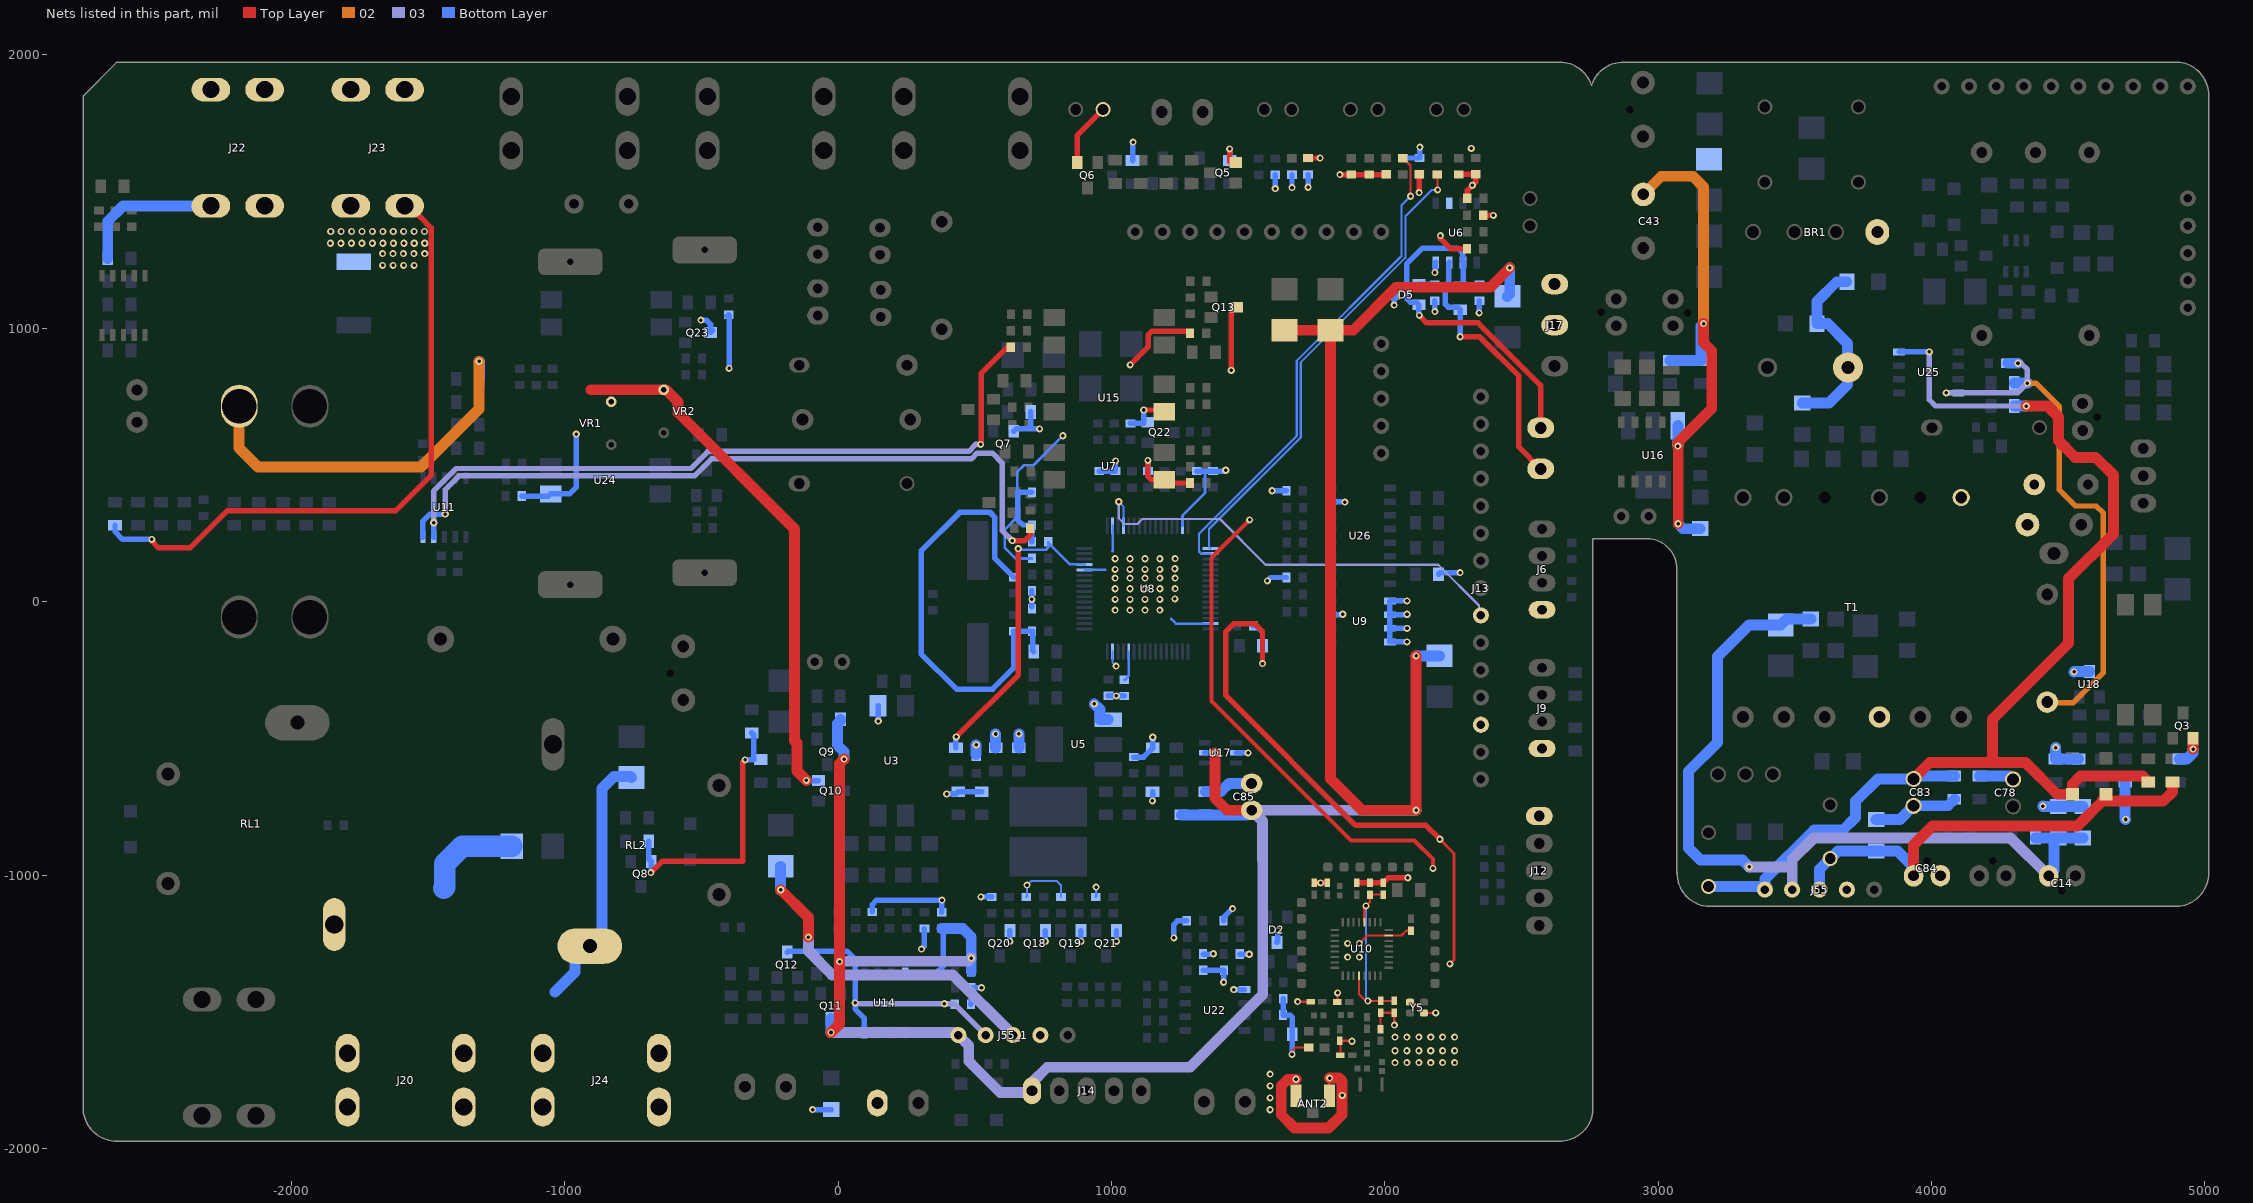
[diagram p0: the nets of this part, all layers, seen from the top]
# Altium PCB MISC105418.PcbDoc (part 3 of 7)
Units mil, origin at the board's own origin, x right, y up, seen from the top; angles counter-clockwise.
Board outline 7774.32 x 3947.04 mil, 4 copper layers (Top Layer, 02, 03, Bottom Layer), stack 30.635 mil thick; 459 components, 285 nets, 1258 pads, 468 vias.
Unrouted connection lines stored in the file: 23.

## Part data
ANT1: library part 天线
BR1: library part BRIDGE1, "Diode Bridge"
C1 C2 C3 C5 C7 C8 C9 C10 C11 C12 C25 C27 C28 C29 C30 C31 C33 C44 C49 C79 C80 C81 C82 C86 C87 C119 C120 CX2 CY1: library part CAP, "Capacitor"
C4 C37 C41 C50 C54 C55 C56 C57 C58 C59 C61 C63 C64 C65 C66 C67 C68 C69 C70 C71 C72 C73 C77 C90 C91 C92 C93 C95 C96 C97 C103 C104 C105 C106 C109 C115 C116 C117 C118: library part CAP/0805, "0.1uF, ,X7R, 10%,50V, SMD"
C6 C13 C14 C36 C43 C62 C78 C83 C84 C85: library part ELECTRO1, "Electrolytic Capacitor"
C15 C20 C22 C26 C32 C40 C45 C46 C48 C111 C125 C127: library part C0805, "0.1uF/50V, X7R,10%, SMD"
C17 C18 C19 C23: library part "Cap Semi", "1uF/50V, X7R,10%, SMD"
C21 C107 C108: library part CAP/0805, "10uF/10V, X7R, 10%,SMD"
C24 C88 C89: library part C0805, "15pF/50V, X7R,10%, SMD"
C38 C101 C112 C123 C124 C129: library part C0805, "1uF/50V, X7R,10%, SMD"
C39 C110: library part C0805, "20pF/50V, X7R,10%, SMD"
C42 C47: library part ELECTRO
C51: library part C0805
C60: library part CAP/0805, "18pF, ,X7R, 10%,50V, SMD"
C74 C76: library part CAP/0603, "0603 SMD ceramic capacitor/ generic footprint"
C98 C99 C100: library part CAP/0805, "33nF, X7R, 10%,SMD"
C102: library part C0805, "2.2uF/50V, X7R,10%, SMD"
C114: library part C0805, "1nF/50V, X7R,10%, SMD"
C121: library part CAP/EC10B, "Electrolytic capacitor 6.8uF/400V / 20% / DIP / horizontal"
CX1: library part CAP_X2, "X capacitor-275AC-224K"
CX3: library part CAP
D2 D5: library part NUP2105L, "NUP2105L,SMD"
D3 D4 D9 D11: library part DIODE
D6 D7 D8 D10 D14 D15 D16 D19 D20 D21 D22 D23 D25 D26 D555: library part DIODE1, "Diode"
D12 D13: library part Diode/SMD2, "SMD diode, 1N4148"
D17 D31: library part Diode/SMD3, "SMD diode: 1N4148"
D24: library part DIODE, "Diode"
D29 D30: library part Diode/SMD2, "SMD diode, US1M"
F1: library part FUSE2, "Fuse"
FB1: library part L3*3*1.5, "SMD ferrite bead"
FB2: library part Inductor
J1 J2 J3 J4 J25: "Connector/2.54mm pitch/1 X 2"
J6 J9: library part XHS-4, "Connector/2.54mm pitch/1 X 4"
J7 J8 J16 J26: library part XHS-2, "Connector/3.81mm pitch/1 X 2"
J11 J20 J21 J22 J23 J24 J28 J29: "Cord connector"
J12 J14: "2.54mm pin header"
J13: library part Header-15,2.54mm, "Header-15,2.54mm"
J15: "Connector/3.81mm pitch/1 X 2"
J55 J55_1 P51 P51_1: library part Header-5.2.54mm, "Header-5.2.54mm"
L1: library part "Ind DR 10x12"
L11 L21 L22 L31: library part L3*3*1.5
L24 L25 L29: library part "INDUCTOR IRON"
L26 L27 L28 L30: library part L3*3*1.5, "SMD inductor"
LF1: library part TRANS6
Q1 Q3: library part NPN1, "NPN Transistor"
Q2: library part "MOSFET N"
Q5 Q6 Q7 Q8 Q10: library part 2N7002, "N-Channel ,AP2306AGN"
Q9 Q14 Q16: library part MOS管P沟道SMD, "P-Channel ,AOSS21311C"
Q11: library part Q-NPN
Q12: library part Q-PNP
Q18 Q19 Q20 Q21 Q22: library part MOS管N沟道SMD, "N-Channel ,AP2306AGN"
R5 R8 R10 R12 R13 R14 R16 R17 R19 R20 R22 R23 R241: library part RES1
R6 R7 R9 R11 R15 R21 R24 R25 R26 R27 R28 R29 R32 R33 R35 R36 R37: library part RES2A, "Resistor"
R18 R141 R142 R156 R159: library part RES/0603
R30 R31 R34: library part RE2A
R38 R39 R45 R88 R92 R95: library part "R 1206_Dup1"
R40 R47 R48 R51 R60 R83 R87 R93 R105 R127 R134 R137 R170 R174 R175 R177 R234 R235 R236 R238: library part RES/0603, "100R,1%,1/10W,SMD"
R41 R125 R126 R213 R214: library part RES/0603, "5.1K,1%,1/10W,SMD"
R42 R43 R113 R114 R116 R117 R119 R120 R121 R122 R151 R153 R155 R157 R158: library part RES/0603, "1K,1%,1/10W,SMD"
R44: library part RES/0805, "1M,1%,1/10W,SMD"
R46 R49 R50 R52 R53 R54 R55 R77 R115 R118 R128 R147 R150 R152 R154 R162 R163 R171 R173 R178 R189 R190 R233 R239 R240 R264: library part RES/0603, "10K,1%,1/10W,SMD"
R56 R57: library part RES/0603, "1K,1%,1/8W,SMD"
R58 R59 R68 R69 R73 R74 R130 R136: library part RES/0603, "10K,1%,1/8W,SMD"
R61 R64 R80 R86 R90 R104 R108 R111 R133: library part RES/0603, "4.7K,1%,1/10W,SMD"
R63 R66 R89 R107 R110: library part RES/0805, "300R,1%,1/8W,SMD"
R65 R85 R91 R109 R112: library part RES/0603, "2K,1%,1/10W,SMD"
R67 R71 R72: library part RES/0603, "470R,1%,1/8W,SMD"
R70 R129 R135: library part RES/0603, "5.1K,1%,1/8W,SMD"
R75: library part RES/0805, "2K,1%,1/8W,SMD"
R78: library part RES/0603, "120K,1%,1/10W,SMD"
R79: library part RES/0603, "1.5K,1%,1/10W,SMD"
R81 R82: library part RES/0603, "20K,1%,1/10W,SMD"
R84: library part RES/0603, "100K,1%,1/10W,SMD"
R94 R102 R185 R186 R187 R231: library part RES/0805, "1.5M,5%,1/8W,SMD"
R96: library part RES/0805, "0R,1%,1/8W,SMD"
R97 R99 R182 R183 R184 R188: library part RES/0805, "1K,1%,1/8W,SMD"
R100: library part RES/0805, "510K,1%,1/8W,SMD"
R103: library part RES/0805, "NC"
R123 R124 R145: library part RES/0805, "3K,5%,1/8W,SMD"
R139 R140 R260 R261: library part RES/0603, "0R,1%,1/10W,SMD"
R148 R149 R191 R192 R193 R194 R197 R199 R201: library part "Res Semi", "Semiconductor Resistor"
R176 R179: library part RES/0603, "100R,1%,1/8W,SMD"
R180 R181: library part RES/0603, "100R,5%,1/8W,SMD"
R195 R198 R200 R263: library part RES/0603, "30K,1%,1W,SMD"
R196: library part RES/0805, "10K, 5%,1/8W, SMD"
R232: library part RES/0805, "1K,5%,1/8W,SMD"
R237: library part RES/0603, "3K,1%,1/10W,SMD"
RL1 RL2: library part HF33F05HSL
RNTC1 RNTC2: library part RES/VARISTOR
T1: library part PQ2020
T2: library part "IND CM T6x3x2"
U1: library part OB2365
U2 U3 U7 U15 U23 U24: library part TLP521-1
U5 U16: library part CM1117, "CM1117"
U9: library part 24LC128
U12: library part DHC05CD4
U14: library part SGM8272, "LM358"
U17: "SM8102H, Pin to Pin"
U18: "Zener Diode"
U20: library part OPTO2A, "Optoisolator"
U22: library part ADM483E
U25: library part LM393D, "Dual Comparator"
U26: library part MAX232ACSE, "+5V Powered, Multi-Channel RS-232 Driver/Receiver"
VR1 VR2: library part RES/VARISTOR, "Varistor, TFMOV10M250"
Y1 Y5: library part CS325
Y2 Y3: library part CAP_X2, "10nF/2KV, X7R, 10%,SMD"
ZC1: library part 放电管
ZD1: library part ZENER1, "Zener Diode"
ZD2 ZD3: library part ZENER2, "Zener Diode"

## Free pads (board coordinates)
  oval 133.86x157.48 hole 125.98: 1(-2191,-56.5) 1(-2191,715) 1(-1932,-56.5) 1(-1932,715)

## Via types
v1: diameter 26, hole 13, Top Layer to Bottom Layer, tented both sides, 468 vias

## Nets (pads, with @x,y where several pads share a name; then routed paths per layer and width w, separated by ;. In a path a pad name is that pad's centre, name@x,y a point inside that pad or via, vN(x,y) a via of type N, cw(c..) or ccw(c..) an arc to the next point about the centre after c; other vN are vias at no path point)
1V2: C102.2 C111.1 C112.1 C127.2 U10.12 U10.28 | length 714.5
  Top Layer w8: U10.28@1905.25,-1368.92 1905.25,-1436.25 1929.79,-1460.79 v1(1938,-1460.79) C111.1@1984.76,-1460.79 C112.1@2034.17,-1460.79 ; U10.12@1924.94,-1172.07 1924.94,-1119.06 v1(1931,-1113) 1945.43,-1098.57 C127.2@1945.43,-1071.49 C102.2@1993.76,-1071.49
  Bottom Layer w8: v1(1931,-1113) 1931,-1453.79 v1(1938,-1460.79)
4GEN/SPI-CS-PA4: J13.9 U8.20 | length 1659.4
  03 w8: v1(1026.47,365.47) 1026.47,304.53 1047,284 1095,284 1113,302 1396.6,302 1563.6,135 2195.18,135 2344.42,-14.24 2344.42,-43.63 J13.9@2351.09,-50.3
  Bottom Layer w8: v1(1026.47,365.47) 1043.51,348.43 U8.20@1043.51,277.82
12VA: C43.1 C44.2 D9.1 L1.2 R95.1 U16.3 | length 1975.7
  Top Layer w39.37: v1(3073,285) 3073,568 v1(3072,569) 3072,582.76 3196,706.76 3196,917.42 3166,947.42 v1(3166,1017)
  02 w39.37: C43.1@2945.36,1490.03 3011.33,1556 3127,1556 3166,1517 v1(3166,1017)
  Bottom Layer w19.68: v1@3071.95,569.05 v1(3072,569)
  Bottom Layer w39.37: L1.2@3042.88,882.44 C44.2@3156,882.44 3156,1007 v1(3166,1017) ; v1@3071.95,569.05 U16.3@3071.95,644.04 ; v1(3073,285) 3091.04,266.96 R95.1@3154,266.96
+6V: C84.1 D15.1 J55.3 J55_1.3 L25.2 R26.1 R34.2 ZD2.2 | length 2907.9
  Top Layer w40: v1(-210,-1054) -109,-1155 v1(-109,-1227) ; C84.1@3934.06,-1002.89 3934.06,-889.94 4003,-821 4533,-821 4624,-730 4847,-730 4881,-696 R26.1@4881,-659.32
  03 w40: v1(-109,-1227) -109,-1278 -22,-1365 419.07,-1365 J55_1.3@639.81,-1585.74
  Bottom Layer w40: v1(-210,-1054) D15.1@-210,-967.8 ; J55.3@3590.09,-1053.5 3590.09,-978.92 L25.2@3629.09,-939.92 3656.96,-912.06 R34.2@3797.09,-912.06 3875.35,-912.06 3934.06,-970.76 C84.1@3934.06,-1002.89
+12.7V: C46.2 C83.1 C85.1 C86.2 C87.2 D7.1 D8.1 D16.1 D555.1 J14.1 J55.1 J55_1.1 L24.2 Q9.2 Q11.3 R28.1 R35.1 R70.1 R75.1 R77.2 R194.1 U14.8 U17.5 U25.8 ZD3.2 | length 14291.5
  Top Layer w39.37: v1(-26,-1576) 5.32,-1544.68 v1(5.32,-1316.88) 5.32,-592.68 v1(22,-576) ; D8.1@1633,993.2 D16.1@1801,993.2 1884.2,993.2 2041,1150 2386,1150 v1(2457,1221)
  Top Layer w40: v1(1379,-553) 1379,-719 1423,-763 C85.1@1513,-763 ; D16.1@1801,993.2 1801,-648 1916,-763 v1(2114,-763) 2114.5,-762.5 v1(2114.5,-198.5) ; C83.1@3933.98,-648.28 3993.26,-589 4206,-589 ; v1(4346,715.53) 4423.47,715.53 4464,675 4464,589 4525,528 4600,528 4665,463 4665,248 4501,84 4501,-152 4223.49,-429.51 4223.49,-571.51 4206,-589 ; R28.1@4793,-659.32 4771.68,-638 4545,-638 4515.09,-667.91 ZD3.2@4515.09,-704.5 4459.39,-704.5 4343.89,-589 4206,-589
  03 w19.68: v1(3991.5,913.5) 3991.5,738.5 4014.47,715.53 v1(4346,715.53)
  03 w39.37: v1(-26,-1576) 430.07,-1576 J55_1.1@439.81,-1585.74 478,-1623.93 478,-1681.33 592.67,-1796 702.47,-1796 J14.1@708.98,-1789.5 708.98,-1759.02 765,-1703 1287,-1703 1553,-1437 1553,-947 ; v1@7.2,-1315 475.94,-1315 v1(486.94,-1304)
  03 w40: 1553,-947 1553,-803 C85.1@1513,-763 v1(2114,-763)
  Bottom Layer w19.68: U25.8@3880.83,913.5 v1(3991.5,913.5)
  Bottom Layer w20: U14.8@245.09,-1359.23 358.77,-1359.23 385,-1333 385,-1201.72 C46.2@378.89,-1195.61 ; U17.5@1340.91,-553 v1(1379,-553)
  Bottom Layer w39.37: v1(-26,-1576) -25.91,-1575.91 Q11.3@-25.91,-1525.22 ; R75.1@5.32,-1360.82 v1(5.32,-1316.88) ; R70.1@8.32,-430 8.32,-435.31 -2.6,-446.24 Q9.2@-2.6,-502.74 -2.6,-524.91 22,-549.5 v1(22,-576) ; C46.2@378.89,-1195.61 455.61,-1195.61 486.94,-1226.94 v1(486.94,-1304) R77.2@486.94,-1353.53 ; D7.1@2448.09,1116.5 2457,1125.41 v1(2457,1221)
  Bottom Layer w40: R35.1@1255.09,-779.82 C86.2@1343.09,-779.82 1496.18,-779.82 C85.1@1513,-763 ; v1(2114.5,-198.5) D555.1@2200.09,-198.5 ; L24.2@3184.09,-1041.92 3378.52,-1041.92 J55.1@3390.09,-1053.5 3390.09,-1014.91 3569,-836 3675,-836 3722,-789 3722,-730 3803.72,-648.28 C83.1@3933.98,-648.28 3944.09,-638.17 C87.2@4083.09,-638.17 ; R194.1@4302.22,715.53 v1(4346,715.53)
+311V: BR1.1 C5.1 C7.2 C62.1 R5.1 R14.1 R201.2 T1.1 | length 704.9
  Bottom Layer w39.37: R201.2@3526.98,726.56 3624.56,726.56 3692,794 3692,944.65 3619.65,1017 C5.1@3580.56,1017 3580.56,1097.56 3653,1170 R5.1@3689.88,1170
-: ANT2.2 C4.2 C15.2 C20.2 C21.2 C22.2 C23.1 C24.1 C25.2 C26.2 C28.2 C29.2 C30.2 C31.2 C32.2 C37.1 C38.1 C39.1 C40.2 C41.1 C45.2 C46.1 C48.2 C54.2 C55.2 C56.1 C57.2 C58.1 C60.1 C61.1 C63.1 C65.2 C66.2 C67.1 C68.1 C69.1 C70.2 C71.2 C72.1 C73.2 C77.2 C78.2 C81.1 C82.2 C83.2 C84.2 C85.2 C86.1 C87.1 C88.2 C89.2 C91.1 C95.2 C97.1 C101.2 C102.1 C103.2 C104.2 C105.2 C106.2 C107.2 C108.2 C109.1 C110.2 C111.2 C112.2 C114.2 C115.1 C116.2 C117.1 C118.1 C119.2 C123.2 C124.2 C125.2 C127.1 C129.2 CY1.1 D2.3 D5.3 FB1.1 J6.4 J9.4 J12.5 J13.13 J16.1 J17.2 J25.1 J55.4 J55_1.4 Q3.2 Q5.2 Q6.2 Q7.2 Q8.2 Q10.2 Q13.3 Q18.2 Q19.2 Q20.2 Q21.2 Q22.2 Q23.3 R27.2 R29.2 R30.2 R31.2 R33.2 R34.1 R37.2 R46.2 R49.2 R50.2 R52.2 R58.1 R59.1 R68.1 R73.1 R74.1 R79.1 R84.1 R113.1 R114.1 R117.1 R120.1 R121.2 R122.2 R128.2 R156.1 R159.1 R171.2 R193.2 R239.2 T1.10 U3.3 U5.1 U6.2 U6.8 U7.3 U8.12 U8.18 U8.31 U8.47 U8.63 U9.1 U9.2 U9.3 U9.4 U9.7 U10.7 U15.3 U17.2 U18.A U22.5 U24.3 U25.4 U26.15 VR1.4 VR2.3 Y5.2 Y5.4 | length 21501.7
  Top Layer w8: v1(1660.28,-1656) 1660.28,-1642.72 1671.78,-1631.22 C125.2@1721.09,-1631.22 ; v1(1681,-1463) 1681.58,-1463.58 C129.2@1728.26,-1463.58 ; C61.1@1826.64,-1465.03 1826.64,-1431.36 v1(1827,-1431) ; C4.2@1837.64,-1659.03 1837.64,-1609.03 C60.1@1835.09,-1606.49 1878.26,-1606.49 v1(1879.77,-1608) ; v1(1907,-1250) 1935.72,-1221.28 U10.7@2013.52,-1221.28 2060.72,-1221.28 2078,-1204 C38.1@2091,-1204 ; C63.1@1984.09,-1563.57 1984.09,-1504.38 C111.2@1984.76,-1503.71 C112.2@2034.17,-1503.71 2034.17,-1548.17 v1(2035,-1549) ; Y5.4@2091.99,-1465.21 2103.8,-1465.21 Y5.2@2143.17,-1504.58 2185.42,-1504.58 v1(2186,-1504)
  Top Layer w10: ANT2.2@1797.02,-1807 1797.02,-1743.98 v1(1798,-1743) ; v1(2201,-869) 2253,-921 2253,-1310 v1(2238,-1325)
  Top Layer w15: v1(1505,299) 1366.57,160.57 1366.57,-364.25 1875.82,-873.5 2107.5,-873.5 2176,-942 v1(2176,-976)
  Top Layer w19.68: Q6.2@874.86,1606.34 874.86,1706.27 J25.1@969.09,1800.5
  Top Layer w20: v1(-685,-991) -643,-949 -349,-949 -349,-588 v1(-340,-579) ; v1(1068,866) 1134.78,932.78 1134.78,976.78 1147,989 1280.11,989 C54.2@1287.2,981.91 ; v1(1118,701) 1186.79,701 U15.3@1192.79,695 ; v1(1133,517) 1133,458 1145,446 U7.3@1192.79,446 1204.79,434 C91.1@1287.2,434 ; v1(1432.09,1655.91) 1432.09,1609.91 1445.06,1596.94 Q5.2@1454.52,1606.4 ; v1(1438,846) 1438,1058.16 Q13.3@1456.75,1076.91 ; v1(1552.44,-226.56) 1552.44,-108.33 1525.12,-81 1447.13,-81 1418.07,-110.07 1418.07,-342.92 1893.15,-818 2150,-818 v1(2201,-869) ; C72.1@1719,1622.87 v1(1762.87,1622.87) ; C123.2@1741.73,-1028.57 v1(1765,-1028.57) C124.2@1789.02,-1028.57 ; v1(1835.37,1562.28) R121.2@1877,1562.28 R156.1@1943,1562.28 C71.2@2005,1562.28 ; C101.2@1897,-1028.57 C127.1@1945.43,-1028.57 C102.1@1993.76,-1028.57 2012.33,-1010 v1(2084,-1010) ; v1(2125.17,1496.17) 2125.58,1496.58 2125.58,1563.04 C89.2@2126,1563.46 ; v1(2203,1339) 2203,1328 2240.05,1290.95 C118.1@2300.46,1290.95 ; R113.1@2270,1562.28 2271.18,1563.46 C117.1@2332,1563.46 2332,1535 2301.65,1504.65 R114.1@2301.65,1476 R114.1@2302.83,1474.82 ; C66.2@2359.91,1413.53 2360.18,1413.27 2396.73,1413.27 v1(2397,1413)
  Top Layer w40: -904,775 VR2.3@-638,775 -630,775 -585,730 -585,691 -160,266 -160,-508.85 -151,-517.85 -151,-619 v1(-116,-654) ; v1(1675,-1747) 1645,-1747 1621,-1771 1621,-1877 1670,-1926 1794,-1926 1844,-1876 v1(1844,-1806) 1844,-1754 1833,-1743 v1(1798,-1743) ; v1(4956.5,-539.5) Q3.2@4956.5,-499.76
  02 w19.68: v1(4350.53,799.53) 4381.47,799.53 4467,714 4467,409 4526,350 4602,350 4628,324 4628,-260 4518,-370 4425.75,-370 CY1.1@4423.09,-367.35
  03 w19.68: v1(4053.5,763.5) 4314.5,763.5 v1(4350.53,799.53) 4350.53,848.47 4327,872 v1(4316,872)
  Bottom Layer w8: R49.2@688.63,-1080.05 691,-1077.68 v1(691,-1037) 706,-1022 800,-1022 815.57,-1037.57 R50.2@815.57,-1080.05 ; R128.2@942.51,-1080.05 944,-1078.55 v1(944,-1044) ; U8.63@1004.14,-182.81 1004.14,-223 1017,-235.86 v1(1017,-236)
  Bottom Layer w10: 655,401.93 655,474 680,499 714,499 v1(822,607) ; 657,311 610,264 610,197 648.78,158.22 C73.2@709.08,158.22 ; U8.12@901.78,116.4 976,116.4 ; 1003,184 1004.14,185.14 U8.18@1004.14,277.82 ; 1219,-63.4 1236.28,-80.68 1362.18,-80.68 U8.47@1362.41,-80.45 ; U8.31@1260.05,277.82 1260.05,315.45 1342.28,397.68 1342.28,472.77 1347.24,477.72
  Bottom Layer w19.68: v1(4053.5,763.5) U25.4@4097.36,763.5
  Bottom Layer w20: C97.1@-1156.98,386.5 -1156.23,385.75 -1112,385.75 ; -1111,386 -1059.82,386 U24.3@-1051.69,394.12 -981.88,394.12 -958,418 v1(-958,613) ; R74.1@-692.8,-876.15 -692.8,-941.03 Q8.2@-683.94,-949.89 -683.94,-989.94 v1(-685,-991) ; v1(-502,1030) -482,1030 -466.5,1014.5 Q23.3@-466.5,984.5 Q23.3@-459.14,991.87 ; C95.2@-407.72,1044.12 -402.56,1049.28 C95.2@-400,1049.28 -399,1048.28 v1(-399,853) ; v1(-340,-579) -338.8,-577.8 -309,-577.8 -309,-487.38 C45.2@-316,-480.38 ; v1(-116,-654) -115.7,-654.3 -72.56,-654.3 Q10.2@-72.26,-654.6 ; v1(-93,-1858) -92.94,-1858.06 FB1.1@-24.91,-1858.06 ; R84.1@125.17,-1134.98 125.17,-1107.83 141,-1092 v1(380,-1092) 378.89,-1093.11 C46.1@378.89,-1136.16 ; U3.3@146.09,-380.71 147,-381.61 v1(147,-437) ; v1(305,-1271) 315.76,-1260.24 C114.2@315.76,-1195.61 ; v1(397.22,-703.57) 398.37,-702.42 432.65,-702.42 C28.2@439.9,-695.17 C30.2@524.9,-695.17 ; C48.2@485.76,-1472.5 486.94,-1471.31 R79.1@486.94,-1412.5 v1(524.5,-1412.5) ; v1(522.31,-1080.05) R52.2@561.69,-1080.05 ; v1(628.38,-1242.62) Q20.2@628.38,-1203.24 ; C39.1@642,89.72 573,158.72 573,308.7 554.7,327 445,327 304,186 304,-191 433,-320 565,-320 642,-243 C110.2@642,-108 642.25,-108.25 711.97,-108.25 712.22,-108.5 712.22,-179.36 C108.2@715.35,-182.5 ; Q7.2@642.4,623.26 651.14,632 702,632 ; R68.1@704.32,694 704.32,634.32 702,632 ; C40.2@709.08,-18.07 C15.2@709.08,40.36 ; C37.1@709.08,218.65 C65.2@709.08,279.08 707.79,280.36 675.64,280.36 657,299 657,311 657,399.93 C70.2@709.08,399.93 ; v1(737,632) 702,632 ; v1(758.38,-1242.62) Q18.2@758.38,-1203.24 ; v1(888.38,-1242.62) Q19.2@888.38,-1203.24 ; C105.2@955,477.72 C55.2@1014.43,477.72 1014.43,514.43 v1(1015,515) ; C104.2@989,-344 989.59,-344.59 1046.41,-344.59 R46.2@1047,-345.18 ; v1(1018.38,-1242.62) Q21.2@1018.38,-1203.24 ; R239.2@1069.36,651.72 1118,651.72 v1(1118,701) ; R59.1@1077.09,1613.34 1078.05,1614.3 1078.05,1680.05 v1(1079,1681) ; C26.2@1081.09,-568.36 1117.37,-568.36 C25.2@1151.09,-534.64 v1(1151.09,-495.91) ; v1(1133,517) 1133.29,516.71 C57.2@1133.29,477.72 ; v1(1149.69,-729) 1150.08,-728.61 R37.2@1150.08,-695.17 ; v1(1228,-1230) 1228,-1181 1241.38,-1167.62 C56.1@1275.45,-1167.62 ; C116.2@1311.57,477.72 1347.24,477.72 C103.2@1371,477.72 1414.96,477.72 v1(1418,480.76) ; C67.1@1334.9,-1289.07 1371.93,-1289.07 v1(1373,-1288) ; R117.1@1336.08,-1348.62 R120.1@1411.18,-1348.62 1411.18,-1390.96 v1(1410,-1392.14) ; C69.1@1410,-1167.62 1410,-1156 v1(1443,-1123) ; R58.1@1432.09,1613.34 v1(1432.09,1655.91) ; v1(1447.04,-1418.96) U22.5@1486.06,-1418.96 ; U17.2@1455.48,-553 v1(1500,-553) ; C58.1@1469.45,-1289.07 1503.07,-1289.07 v1(1504,-1290) ; C106.2@1518.72,-88 1528.89,-88 1552.44,-111.56 C107.2@1552.44,-161 v1(1552.44,-226.56) ; v1(1570,76) 1582.29,88.29 C41.1@1640.19,88.29 ; v1(1587.3,405.7) C20.2@1640.19,405.7 ; v1(1599.09,1510.91) R122.2@1599.09,1561.24 ; D2.3@1605.2,-1246.76 1607.85,-1244.1 1607.85,-1204.15 v1(1609,-1203) ; R171.2@1628.76,-1452.14 1627.58,-1453.32 C22.2@1627.58,-1512.14 1653.14,-1512.14 1661.3,-1520.3 C21.2@1661.3,-1582.14 1661.3,-1654.98 v1(1660.28,-1656) ; v1(1660.28,1514.28) R159.1@1660.28,1561.24 ; v1(1719.09,1515.91) C77.2@1719.09,1562.42 ; U9.7@1801.83,-47.42 1844.58,-47.42 v1(1846,-46) ; U26.15@1801.83,365.7 1852.3,365.7 v1(1854,364) ; D5.3@2031.74,1123.43 2034,1121.17 v1(2034,1085) ; C68.1@2065.9,1622.91 C115.1@2128.17,1622.91 v1(2128.17,1662.83) ; v1@2078,-97.42 v1@2078.58,-98 ; v1@2078,-47.42 v1@2079.42,-46 ; v1@2078,2.58 v1@2078.42,3 ; v1@2080.58,2.58 U9.1@2018.36,2.58 U9.2@2018.36,-47.42 ; v1@2084,-147.42 U9.4@2018.36,-147.42 U9.3@2018.36,-97.42 ; v1@2085.58,-47.42 U9.2@2018.36,-47.42 ; v1@2086.42,-97.42 U9.3@2018.36,-97.42 ; v1(2183,1061) C24.1@2183,1101.04 ; v1(2183,1204) 2184.15,1205.15 2184.15,1239.01 U6.8@2186.09,1240.96 ; C23.1@2196.42,100.7 2201.72,106 v1(2275,106) ; v1(2345,1056) 2345.55,1056.55 2345.55,1100.5 C88.2@2346.09,1101.04 ; U9.3@2018.36,-97.42 U9.2@2018.36,-47.42
  Bottom Layer w40: C32.2@505.11,-559 v1(505.11,-524.11) ; C31.2@576.09,-534.64 v1(576.09,-484.09) ; C29.2@661.09,-534.64 v1(661.09,-483.91) ; v1(937,-374) 958,-395 958,-431.55 U5.1@988.09,-431.55 ; C86.1@1343.09,-695.17 1399.83,-695.17 1430.03,-664.97 C85.2@1512.61,-664.97 ; R34.1@3797.09,-796.94 3883.75,-796.94 C83.2@3933.98,-746.71 4059.2,-746.71 C87.1@4083.09,-722.82 ; C81.1@4175.09,-638.17 4285.77,-638.17 C78.2@4298.09,-650.5 ; C119.2@4279,872 v1(4316,872) ; R193.2@4302.22,799.53 v1(4350.53,799.53) ; v1(4407,-748) 4408.11,-749.11 R30.2@4463.09,-749.11 R31.2@4553.09,-749.11 ; v1(4454,-534) 4453.09,-534.91 R29.2@4453.09,-575.85 R27.2@4538.09,-575.85 ; v1(4521,-257) 4521.76,-256.24 U18.A@4577.09,-256.24 ; C82.2@4708.09,-660.5 4708.09,-795.03 v1(4710,-796.94) ; R33.2@4906,-575.68 4934.32,-575.68 4956.5,-553.5 v1(4956.5,-539.5)
  other v1: 1580,-1858.8 1580,-1815.2 1580,-1771.6 1580,-1728 2037,-1686 2080.6,-1686 2124.2,-1686 2167.8,-1686 2211.4,-1686 2255,-1686 2037,-1643 2080.6,-1643 2124.2,-1643 2167.8,-1643 2211.4,-1643 2255,-1643 2037,-1593 2080.6,-1593 2124.2,-1593 2167.8,-1593 2211.4,-1593 2255,-1593 1864,-1300 1907,-1300 1864,-1250 1018,-344.59 2081,-147.42 2081,-98 2081,-46 1013,-31 1067.75,-31 1122.5,-31 1177.25,-31 2081,3 709.08,8 1013,8 1067.75,8 1122.5,8 1177.25,8 1231.74,10.26 1013,47 1067.75,47 1122.5,47 1177.25,47 1233,47.5 1013,86 1067.75,86 1122.5,86 1177.25,86 1233,86 1013,118 1067.75,118 1122.5,118 1177.25,118 1231.74,120.26 1013,157 1067.75,157 1122.5,157 1177.25,157 1233,157.5 2320,1523 2316,1658
-12.7V: C11.2 C14.2 C48.1 C79.1 D26.1 J17.3 J55.2 J55_1.2 Q12.3 R30.1 R31.1 U14.4 | length 4124.2
  03 w20: v1(62,-1467.5) 63.62,-1467.5 67.13,-1471 v1(389,-1471) 425.07,-1471 J55_1.2@539.81,-1585.74
  03 w40: v1(3333,-970.5) 3487.6,-970.5 3490.09,-968 ; J55.2@3490.09,-1053.5 3490.09,-968 ; C14.2@4428.08,-1002.88 4289.2,-864 3570,-864 3490.09,-943.91 3490.09,-968
  Bottom Layer w20: Q12.3@-185.91,-1282.02 -181.97,-1278.08 32.08,-1278.08 62,-1308 v1(62,-1467.5) 62,-1490 95.09,-1523.09 U14.4@95.09,-1575.76 ; v1(389,-1471) 389.75,-1471.75 425.56,-1471.75 C48.1@426.31,-1472.5
  Bottom Layer w40: v1(3333,-970.5) 3307.5,-945 3155,-945 3111,-901 3111,-620.56 3217,-514.56 3217,-200 3331.47,-85.53 D26.1@3448.09,-85.53 3470.22,-63.4 C11.2@3558.09,-63.4 ; C79.1@4380.02,-863.75 4380.5,-864.23 R30.1@4463.09,-864.23 ; C14.2@4428.08,-1002.88 4447,-983.96 4447,-880.32 R30.1@4463.09,-864.23 ; R31.1@4553.09,-864.23 R30.1@4463.09,-864.23
A3.3V: C37.2 L31.2 U8.13 | length 1113.2
  Top Layer w20: v1(432,-495) 659,-268 v1(659,194.31)
  Bottom Layer w10: v1(659,194.31) 663.38,189.93 760.93,189.93 768.53,197.53 C37.2@768.53,206.53 ; C37.2@768.53,216.09 848.21,136.4 901.46,136.4 U8.13@901.78,136.09
  Bottom Layer w20: L31.2@431.09,-534.64 431.09,-495.91 v1(432,-495)
ACL-IN: J22.1 pad.1@-2191,715 R185.2 R231.2 | length 1922.6
  02 w40: pad.1@-2191,715 -2191,561.81 -2121.97,492.79 -1525.21,492.79 -1313,705 v1(-1313,879)
  Bottom Layer w40: R185.2@-2671.55,1255.67 -2671.55,1391.45 -2615.18,1447.82 J22.1@-2294.43,1447.82 ; v1(-1313,879) -1312.47,878.47 R231.2@-1312.47,814.53
ACL-OUT: D29.1 J20.1 RL1.4 | length 363.4
  Bottom Layer w78.74: -1443,-1049 -1439,-1045 -1439,-959 -1375,-895 D29.1@-1193.8,-895
ACN-IN: J23.1 R183.1 R184.1 | length 2283.5
  Top Layer w20: v1(-2510,228) -2510,220.99 -2486.01,197 -2370,197 -2235,332 -1619,332 -1489,462 -1489,1367 -1532,1410
  Bottom Layer w20: R184.1@-2645.15,279.31 -2645.15,256.15 -2617,228 v1(-2510,228)
  other v1: -1666,1230 -1627.67,1230 -1589.33,1230 -1551,1230 -1666.33,1273 -1628.22,1273 -1590.11,1273 -1552,1273 -1512,1273 -1857,1311 -1818.67,1311 -1780.33,1311 -1742,1311 -1703.67,1311 -1665.33,1311 -1627,1311 -1588.67,1311 -1550.33,1311 -1512,1311 -1856,1354 -1817.89,1354 -1779.78,1354 -1741.67,1354 -1703.56,1354 -1665.44,1354 -1627.33,1354 -1589.22,1354 -1551.11,1354 -1513,1354
ACN-OUT: D30.2 J24.1 RL2.1 | length 974
  Bottom Layer w40: -1035.77,-1427.9 -962.96,-1355.09 -962.96,-1301.67 -917.42,-1256.14 -864,-1256.14 -864,-684 -820,-640 -759.38,-640 D30.2@-756,-643.38
BL-RX5: R85.2 U11.10 | length 2746.5
  Top Layer w20: v1(637,223) 637.31,223.31 671.01,223.31 671.32,223 682.91,223 703.34,243.44 R85.2@703.34,268
  03 w20: v1(-1437,320) -1437,410.23 -1387.26,459.97 -525.03,459.97 -462.98,522.02 487.07,522.02 508.06,543 564,543 601,506 601,259 v1(637,223)
  Bottom Layer w20: U11.10@-1518.65,236.24 -1518.65,294.35 -1493,320 v1(-1437,320)
BL-TX5: R40.2 U11.9 | length 2647.7
  Top Layer w20: v1(521,575) 523,577 523,834 619.81,930.81 R40.2@631.44,930.81
  03 w20: v1(-1479.28,288.72) -1479.28,404.72 -1397,487 -538.72,487 -476.22,549.5 467,549.5 467.5,550 478,550 503,575 v1(521,575)
  Bottom Layer w20: U11.9@-1479.28,236.24 v1(-1479.28,288.72)
BOOT0: R46.1 U8.60 | length 111.1
  Bottom Layer w10: R46.1@1047,-285.73 1049.56,-285.73 1059.72,-275.57 1059.72,-273.02 1063.2,-269.54 U8.60@1063.2,-182.81
CAN1-H: C24.2 D5.1 J8.2 R179.1 U6.7 | length 1066.8
  Top Layer w20: v1(2275,969) 2347,969 2490,826 2490,565.8 J8.2@2570.09,485.7
  Bottom Layer w20: D5.1@2124.26,1160.83 2124.43,1160.66 2182.83,1160.66 C24.2@2183,1160.49 2185.49,1158 2221,1158 ; U6.7@2236.09,1240.96 2233.89,1238.76 2233.89,1170.89 2221,1158 ; v1(2275,969) 2276.09,970.09 R179.1@2276.09,1067.32 2266.41,1077.01 2232.72,1077.01 2221,1088.72 2221,1158
CAN1-L: C88.1 D5.2 J8.1 R179.2 U6.6 | length 1356.4
  Top Layer w20: v1(2126,1047) 2153,1020 2341,1020 2570.09,790.91 J8.1@2570.09,635.7
  Bottom Layer w20: v1(2126,1047) 2124.26,1048.74 D5.2@2124.26,1086.02 2114.58,1095.71 2093.29,1095.71 2080,1109 2080,1235 2138,1293 2267,1293 2284.42,1275.58 2284.42,1242.63 U6.6@2286.09,1240.96 2286.09,1161.65 R179.2@2280.67,1156.23 ; R179.2@2276.09,1151.97 2280.36,1156.23 R179.2@2280.67,1156.23 ; C88.1@2346.09,1160.49 2341.83,1156.23 R179.2@2280.67,1156.23
CAN2-RX-PB12: R181.2 U8.33 | length 1728.4
  Top Layer w8: R181.2@2192,1562.28 2193,1561.28 v1(2193,1506)
  Bottom Layer w8: U8.33@1362.41,195.14 1357,200.55 1357,265.4 1692,600.4 1692,875.28 2075,1258.28 2075,1409 2172,1506 v1(2193,1506)
CAN2-TX-PB13: R180.2 U8.34 | length 1818.2
  Top Layer w8: R180.2@2065,1621.72 2067.56,1621.72 2094,1595.28 v1(2094,1483)
  Bottom Layer w8: U8.34@1362.41,175.46 1327.77,175.46 1320,183.23 1320,248.2 1678,606.2 1678,881.08 2061,1264.08 2061,1450 v1(2094,1483)